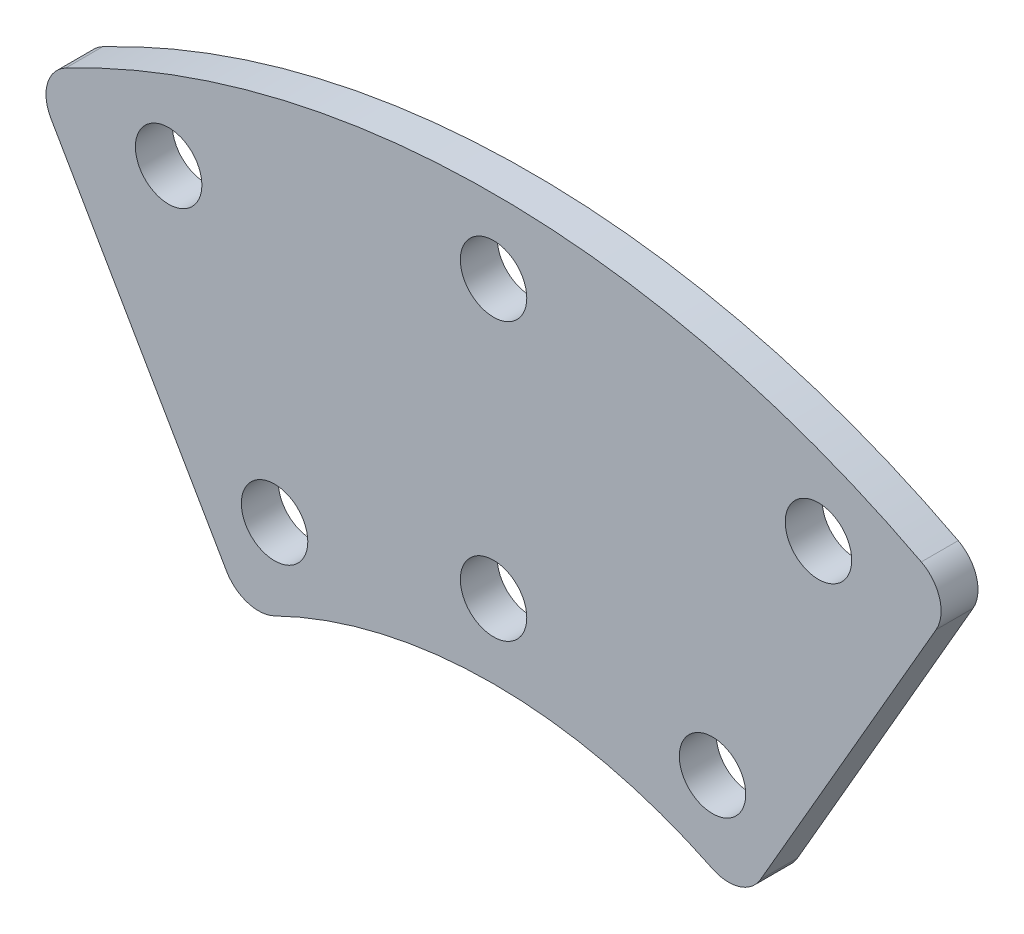
SolidWorks part; units mm, degrees
material "Q235-A "
ref_plane "前视基准面" through (0, 0, 0) normal (0, 0, 1) x (1, 0, 0)
ref_plane "上视基准面" through (0, 0, 0) normal (0, 1, 0) x (1, 0, 0)
ref_plane "右视基准面" through (0, 0, 0) normal (1, 0, 0) x (0, 0, -1)
sketch "草图1" plane through (0, 0, 0) normal (0, 0, 1) x (1, 0, 0)
  line L0 (-59.3159, 143.2013) -> (0, 0) construction
  line L1 (0, 0) -> (59.3159, 143.2013) construction
  line L2 (0, 155) -> (0, 0) construction
  line L3 (-67.5, 116.9134) -> (-125, 216.5064)
  line L4 (67.5, 116.9134) -> (125, 216.5064)
  line L5 (0, 0) -> (67.5, 116.9134) construction
  line L6 (-67.5, 116.9134) -> (0, 0) construction
  circle A0 centre (0, 0) radius 175 construction
  circle A1 centre (0, 0) radius 155 construction
  circle A2 centre (0, 155) radius 9
  circle A3 centre (59.3159, 143.2013) radius 9
  circle A17 centre (-59.3159, 143.2013) radius 9
  circle A18 centre (109.6016, 109.6016) radius 9 [skipped]
  circle A19 centre (143.2013, 59.3159) radius 9 [skipped]
  circle A20 centre (155, 0) radius 9 [skipped]
  circle A21 centre (143.2013, -59.3159) radius 9 [skipped]
  circle A22 centre (109.6016, -109.6016) radius 9 [skipped]
  circle A23 centre (-155, 0) radius 9 [skipped]
  circle A24 centre (-143.2013, 59.3159) radius 9 [skipped]
  circle A25 centre (-109.6016, 109.6016) radius 9 [skipped]
  circle A26 centre (59.3159, -143.2013) radius 9 [skipped]
  circle A27 centre (0, -155) radius 9 [skipped]
  circle A28 centre (-59.3159, -143.2013) radius 9 [skipped]
  circle A29 centre (-109.6016, -109.6016) radius 9 [skipped]
  circle A30 centre (-143.2013, -59.3159) radius 9 [skipped]
  arc A31 (67.5, 116.9134) -> (-67.5, 116.9134) centre (0, 0) ccw
  arc A32 (125, 216.5064) -> (-125, 216.5064) centre (0, 0) ccw
  dimension "D1" = 22.5
  dimension "D2" = 310
  dimension "D3" = 18
  dimension "D6" = 350
  dimension "D7" = 270
  dimension "D9" = 500
  dimension "D5" = 45
  dimension "D8" = 30
  dimension "D10" = 30
  dimension "D4" = 16
extrude "凸台-拉伸1" add sketch "草图1" along normal blind 10
fillet "圆角1" radius 10 4 edges at (125, 216.5064, 5) (67.5, 116.9134, 5) (-67.5, 116.9134, 5) (-125, 216.5064, 5)
sketch "草图2" plane through (0, 0, 10) normal (0, 0, 1) x (1, 0, 0)
  line L0 (0, 0) -> (88.0172, 212.4923) construction
  line L1 (0, 0) -> (0, 230) construction
  circle A0 centre (0, 0) radius 230 construction
  circle A1 centre (0, 230) radius 9
  circle A2 centre (88.0172, 212.4923) radius 9
  circle A3 centre (-88.0172, 212.4923) radius 9
  dimension "D1" = 460
  dimension "D2" = 18
  dimension "D4" = 18
  dimension "D3" = 22.5
extrude "切除-拉伸1" cut sketch "草图2" against normal through all
